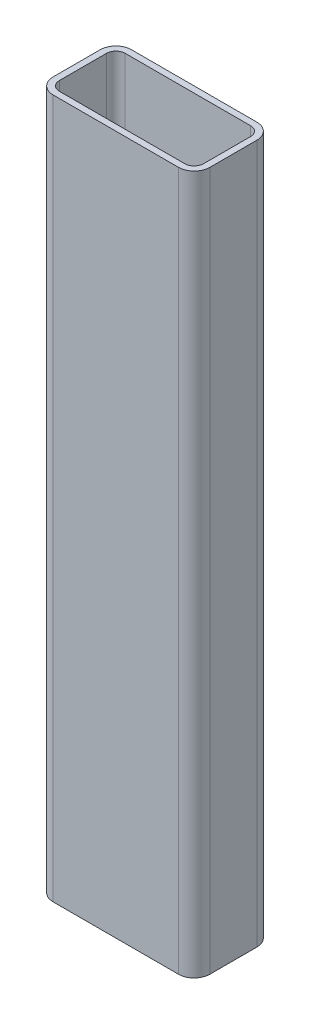
SolidWorks part; units mm, degrees
ref_plane "Front Plane" through (0, 0, 0) normal (0, 0, 1) x (1, 0, 0)
ref_plane "Top Plane" through (0, 0, 0) normal (0, 1, 0) x (1, 0, 0)
ref_plane "Right Plane" through (0, 0, 0) normal (1, 0, 0) x (0, 0, -1)
other "Configuration Table"
sketch "Sketch1" plane through (0, 0, 0) normal (0, 1, 0) x (1, 0, 0)
  line L1 (-40, 25) -> (40, 25)
  line L2 (-50, 15) -> (-50, -15)
  line L3 (-40, -25) -> (40, -25)
  line L4 (50, 15) -> (50, -15)
  line L5 (-50, 25) -> (50, -25) construction
  line L6 (-50, -25) -> (50, 25) construction
  arc A0 (40, 25) -> (50, 15) centre (40, 15) cw
  arc A1 (40, -25) -> (50, -15) centre (40, -15) ccw
  arc A2 (-50, -15) -> (-40, -25) centre (-40, -15) ccw
  arc A3 (-40, 25) -> (-50, 15) centre (-40, 15) ccw
  point P0 (0, 0)
  dimension "D3" = 10
  dimension "D1" = 100
  dimension "D2" = 50
extrude "Extrude-Thin1" add sketch "Sketch1" along normal mid plane 446 thin
